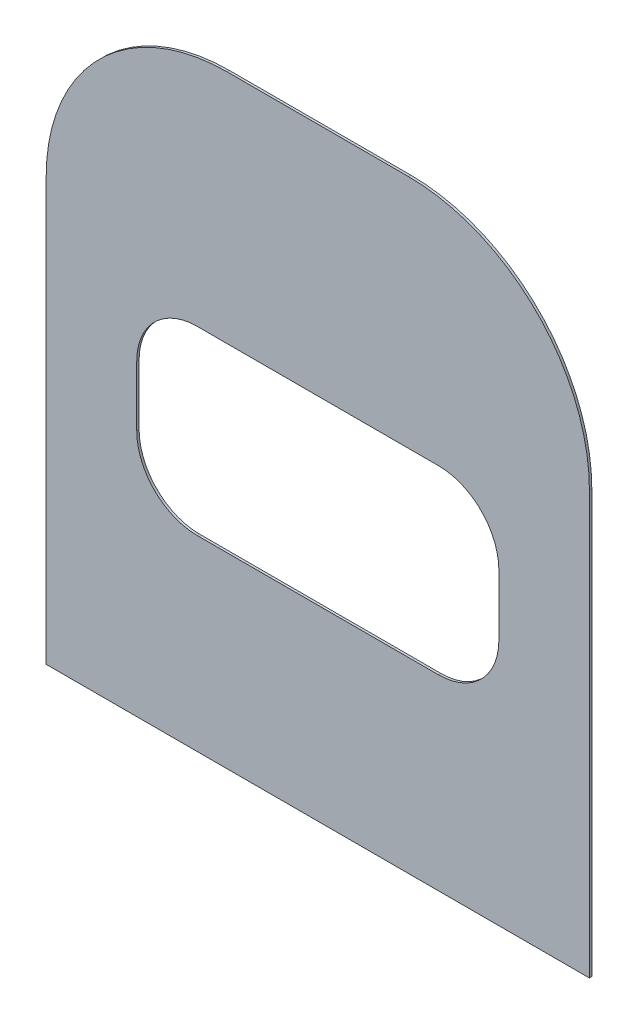
from build123d import *

# Parameters (mm, degrees)
BOSS_EXTRUDE1_DEPTH = 1


with BuildPart() as part:
    # Sketch1 → Boss-Extrude1 (new, symmetric)
    with BuildSketch(Plane.XY):
        with BuildLine():
            Line((-76.2, 508), (76.2, 508))
            ThreePointArc((76.2, 508), (183.963073453, 463.363073453), (228.6, 355.6))
            Line((228.6, 355.6), (228.6, 0))
            Line((228.6, 0), (-228.6, 0))
            Line((-228.6, 0), (-228.6, 355.6))
            ThreePointArc((-228.6, 355.6), (-183.963073453, 463.363073453), (-76.2, 508))
        make_face()
        with BuildLine():
            Line((-101.6, 309.88), (101.6, 309.88))
            ThreePointArc((101.6, 309.88), (137.521024484, 295.001024484), (152.4, 259.08))
            Line((152.4, 259.08), (152.4, 208.28))
            ThreePointArc((152.4, 208.28), (137.521024484, 172.358975516), (101.6, 157.48))
            Line((101.6, 157.48), (-101.6, 157.48))
            ThreePointArc((-101.6, 157.48), (-137.521024484, 172.358975516), (-152.4, 208.28))
            Line((-152.4, 208.28), (-152.4, 259.08))
            ThreePointArc((-152.4, 259.08), (-137.521024484, 295.001024484), (-101.6, 309.88))
        make_face(mode=Mode.SUBTRACT)
    extrude(amount=BOSS_EXTRUDE1_DEPTH, both=True)


solid = part.part
